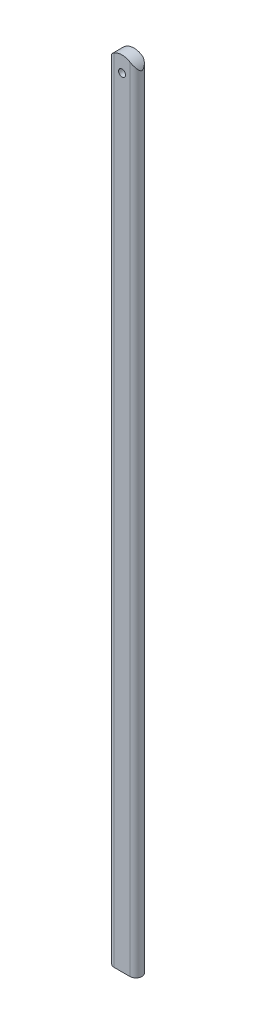
SolidWorks part; units mm, degrees
ref_plane "Front Plane" through (0, 0, 0) normal (0, 0, 1) x (1, 0, 0)
ref_plane "Top Plane" through (0, 0, 0) normal (0, 1, 0) x (1, 0, 0)
ref_plane "Right Plane" through (0, 0, 0) normal (1, 0, 0) x (0, 0, -1)
other "Configuration Table"
sketch "Sketch1" plane through (0, 0, 0) normal (0, 1, 0) x (1, 0, 0)
  line L0 (0, 0) -> (8, 0) construction
  line L1 (0, 3) -> (8, 3)
  line L2 (0, -3) -> (8, -3)
  arc A0 (0, 3) -> (0, -3) centre (0, 0) ccw
  arc A1 (8, -3) -> (8, 3) centre (8, 0) ccw
  point P3 (4, 0)
  dimension "D2" = 3
  dimension "D1" = 8
extrude "Boss-Extrude1" add sketch "Sketch1" against normal blind 400
sketch "Sketch2" plane through (0, 0, -3) normal (0, 0, -1) x (-1, 0, 0)
  line L0 (-4, 0) -> (-4, -15) construction
  line L1 (-8, 0) -> (0, 0) construction
  line L3 (9.5958, 3.0552) -> (9.5958, -10.1233)
  line L4 (9.5958, -10.1233) -> (3.0263, -10.1233)
  line L5 (-18.139, -10.1233) -> (-18.139, 3.0552)
  line L7 (-18.139, 3.0552) -> (9.5958, 3.0552)
  line L8 (-11.0263, -10.1233) -> (-18.139, -10.1233)
  arc A0 (3.0263, -10.1233) -> (-11.0263, -10.1233) centre (-4, -7.5) ccw
  dimension "D1" = 15
extrude "Cut-Extrude1" cut sketch "Sketch2" against normal through all
sketch "Sketch3" plane through (0, 0, 3) normal (0, 0, 1) x (1, 0, 0)
  line L0 (4, 0) -> (4, -11.1411) construction
  arc A0 (8, -1.1557) -> (0, -1.1557) centre (4, -7.5) ccw construction
  circle A1 centre (4, -7.884) radius 1.75
  dimension "D1" = 3.5
extrude "Cut-Extrude2" cut sketch "Sketch3" against normal through all
